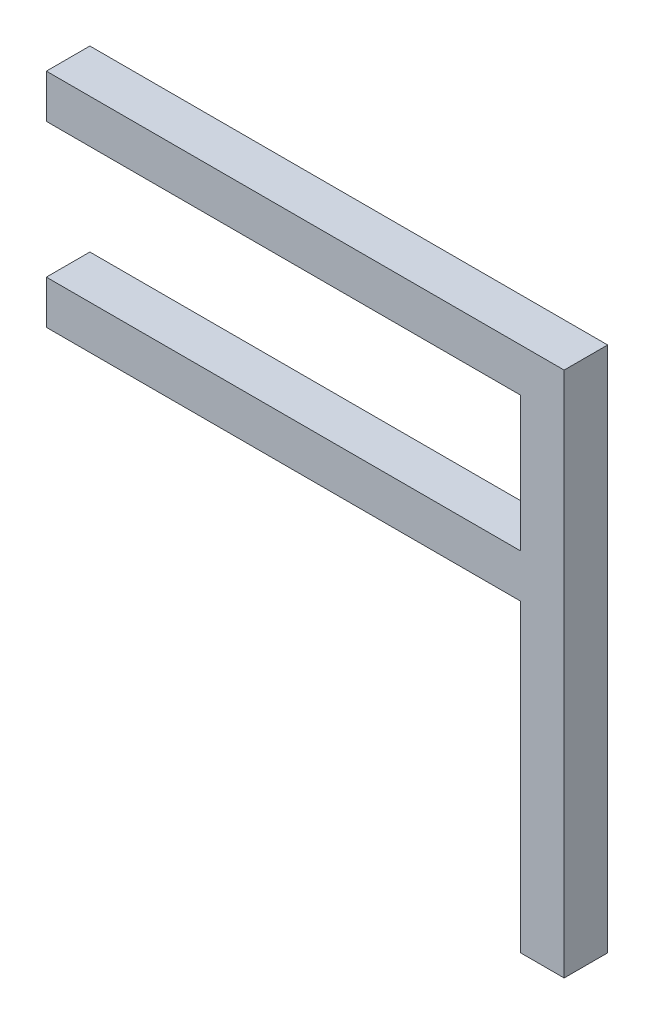
from build123d import *

# Parameters (mm, degrees)
SKETCH_1_W          = 570
SKETCH_1_H          = 545
SKETCH_1_W_2        = 470
SKETCH_1_H_2        = 445
EXTRUDE_1_DEPTH     = 50
SKETCH_2_W          = 470
SKETCH_2_H          = 50
EXTRUDE_2_DEPTH     = 50
SKETCH_3_W          = 50
SKETCH_3_H          = 50
EXTRUDE_3_DEPTH     = 50
SKETCH_4_W          = 470
SKETCH_4_H          = 50
CUT_EXTRUDE_1_DEPTH = 50
EXTRUDE_4_DEPTH     = 478
SKETCH_6_W          = 570
SKETCH_6_H          = 50
CUT_EXTRUDE_2_DEPTH = 76
SKETCH_7_W          = 50
SKETCH_7_H          = 545
EXTRUDE_5_DEPTH     = 50
SKETCH_8_W          = 50
SKETCH_8_H          = 545
CUT_EXTRUDE_3_DEPTH = 50
SKETCH_9_W          = 50
SKETCH_9_H          = 50
EXTRUDE_6_DEPTH     = 20
SKETCH_10_W         = 50
SKETCH_10_H         = 50
EXTRUDE_7_DEPTH     = 10
SKETCH_11_W         = 50
SKETCH_11_H         = 50
EXTRUDE_8_DEPTH     = 60
SKETCH_12_W         = 50
SKETCH_12_H         = 50
EXTRUDE_9_DEPTH     = 45


with BuildPart() as part:
    # 草图1 → 凸台-拉伸1 (new body)
    with BuildSketch(Plane.XY):
        with Locations((285, 272.5)):
            Rectangle(SKETCH_1_W, SKETCH_1_H)
        with Locations((285, 272.5)):
            Rectangle(SKETCH_1_W_2, SKETCH_1_H_2, mode=Mode.SUBTRACT)
    extrude(amount=EXTRUDE_1_DEPTH)

    # 草图2 → 凸台-拉伸2 (add)
    with BuildSketch(Plane(origin=(0, 0, 0), x_dir=(-1, 0, 0), z_dir=(0, 0, -1))):
        with Locations((-285, 315)):
            Rectangle(SKETCH_2_W, SKETCH_2_H)
    extrude(amount=-EXTRUDE_2_DEPTH)

    # 草图3 → 凸台-拉伸3 (add)
    with BuildSketch(Plane.XZ):
        with Locations((25, 25)):
            Rectangle(SKETCH_3_W, SKETCH_3_H)
        with Locations((545, 25)):
            Rectangle(SKETCH_3_W, SKETCH_3_H)
    extrude(amount=EXTRUDE_3_DEPTH)

    # 草图4 → 切除-拉伸1 (cut)
    with BuildSketch(Plane.XY.offset(50)):
        with Locations((285, 25)):
            Rectangle(SKETCH_4_W, SKETCH_4_H)
    extrude(amount=-CUT_EXTRUDE_1_DEPTH, mode=Mode.SUBTRACT)

    # 草图5 → 凸台-拉伸4 (add)
    with BuildSketch(Plane.ZY.offset(-520)):
        Polygon((50, -50), (0, -50), (0, 0), (50, 0), (50, -10.325702711), align=None)
    extrude(amount=EXTRUDE_4_DEPTH)

    # 草图6 → 切除-拉伸2 (cut)
    with BuildSketch(Plane.XY.offset(50)):
        with Locations((285, -25)):
            Rectangle(SKETCH_6_W, SKETCH_6_H)
    extrude(amount=-CUT_EXTRUDE_2_DEPTH, mode=Mode.SUBTRACT)

    # 草图7 → 凸台-拉伸5 (add)
    with BuildSketch(Plane.ZY):
        with Locations((25, 272.5)):
            Rectangle(SKETCH_7_W, SKETCH_7_H)
    extrude(amount=-EXTRUDE_5_DEPTH)

    # 草图8 → 切除-拉伸3 (cut)
    with BuildSketch(Plane.ZY):
        with Locations((25, 272.5)):
            Rectangle(SKETCH_8_W, SKETCH_8_H)
    extrude(amount=-CUT_EXTRUDE_3_DEPTH, mode=Mode.SUBTRACT)

    # 草图9 → 凸台-拉伸6 (add)
    with BuildSketch(Plane.ZY.offset(-50)):
        with Locations((25, 520)):
            Rectangle(SKETCH_9_W, SKETCH_9_H)
        with Locations((25, 315)):
            Rectangle(SKETCH_9_W, SKETCH_9_H)
    extrude(amount=EXTRUDE_6_DEPTH)

    # 草图10 → 凸台-拉伸7 (add)
    with BuildSketch(Plane.ZY.offset(-30)):
        with Locations((25, 520)):
            Rectangle(SKETCH_10_W, SKETCH_10_H)
        with Locations((25, 315)):
            Rectangle(SKETCH_10_W, SKETCH_10_H)
    extrude(amount=EXTRUDE_7_DEPTH)

    # 草图11 → 凸台-拉伸8 (add)
    with BuildSketch(Plane.XZ):
        with Locations((545, 25)):
            Rectangle(SKETCH_11_W, SKETCH_11_H)
    extrude(amount=EXTRUDE_8_DEPTH)

    # 草图12 → 凸台-拉伸9 (add)
    with BuildSketch(Plane.ZY.offset(-20)):
        with Locations((25, 520)):
            Rectangle(SKETCH_12_W, SKETCH_12_H)
        with Locations((25, 315)):
            Rectangle(SKETCH_12_W, SKETCH_12_H)
    extrude(amount=EXTRUDE_9_DEPTH)


solid = part.part
